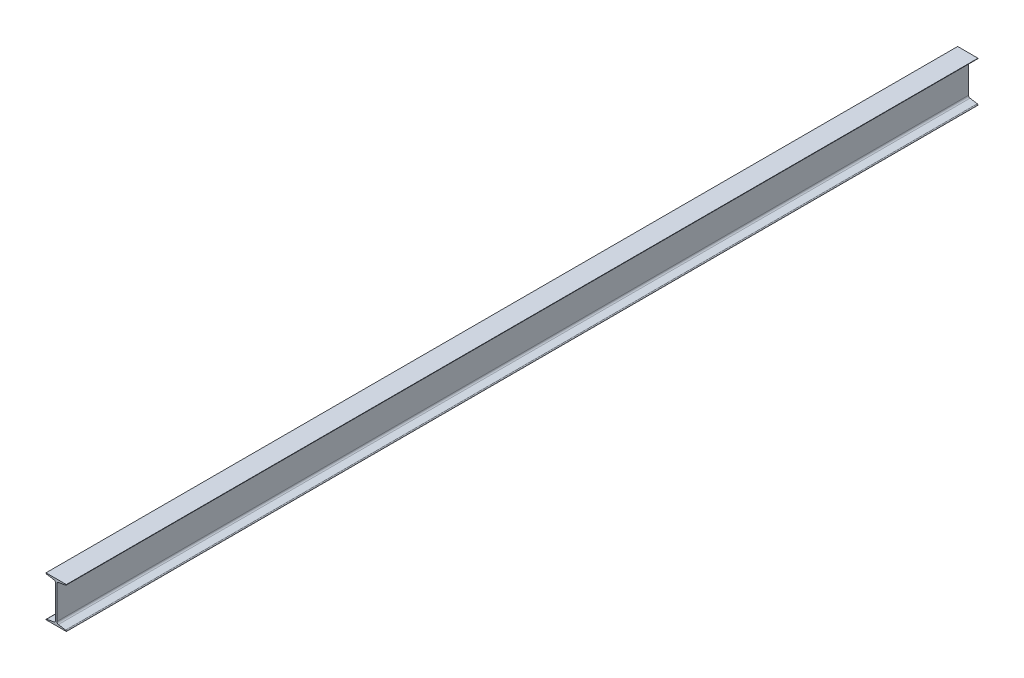
SolidWorks part; units mm, degrees
ref_plane "Front" through (0, 0, 0) normal (0, 0, 1) x (1, 0, 0)
ref_plane "Top" through (0, 0, 0) normal (0, 1, 0) x (1, 0, 0)
ref_plane "Right" through (0, 0, 0) normal (1, 0, 0) x (0, 0, -1)
sketch "Sketch1" plane through (0, 0, 0) normal (0, 0, 1) x (1, 0, 0)
  line L0 (314.4046, 42.2016) -> (314.4046, -38.6137)
  line L1 (307.4046, 42.2016) -> (307.4046, -38.6137)
  line L2 (310.9046, -57.7984) -> (360.9046, -57.7984)
  line L3 (299.8839, -47.4913) -> (264.665, -53.3596)
  line L4 (310.9046, -57.7984) -> (260.9046, -57.7984)
  line L5 (321.9254, -47.4913) -> (357.1442, -53.3596)
  line L6 (307.4046, 42.2016) -> (307.4046, 123.0169)
  line L7 (314.4046, 42.2016) -> (314.4046, 123.0169)
  line L8 (310.9046, 142.2016) -> (360.9046, 142.2016)
  line L9 (299.8839, 131.8945) -> (264.665, 137.7628)
  line L10 (310.9046, 142.2016) -> (260.9046, 142.2016)
  line L11 (321.9254, 131.8945) -> (357.1442, 137.7628)
  arc A0 (321.9254, 131.8945) -> (314.4046, 123.0169) centre (323.4046, 123.0169) ccw
  arc A1 (307.4046, 123.0169) -> (299.8839, 131.8945) centre (298.4046, 123.0169) ccw
  arc A2 (264.665, -53.3596) -> (260.9046, -57.7984) centre (265.4046, -57.7984) ccw
  arc A3 (299.8839, -47.4913) -> (307.4046, -38.6137) centre (298.4046, -38.6137) ccw
  arc A4 (314.4046, -38.6137) -> (321.9254, -47.4913) centre (323.4046, -38.6137) ccw
  arc A5 (360.9046, -57.7984) -> (357.1442, -53.3596) centre (356.4046, -57.7984) ccw
  arc A6 (260.9046, 142.2016) -> (264.665, 137.7628) centre (265.4046, 142.2016) ccw
  arc A7 (357.1442, 137.7628) -> (360.9046, 142.2016) centre (356.4046, 142.2016) ccw
extrude "Boss-Extrude1" add sketch "Sketch1" along normal blind 3580
other "Move Face1" face at (310.9046, 42.2016, 0) parameters "D1"=900
equation "\"零件重量\"= IIF ( \"SW-质量\" > 100 , int ( \"SW-质量\" ) , \"SW-质量\" )"
